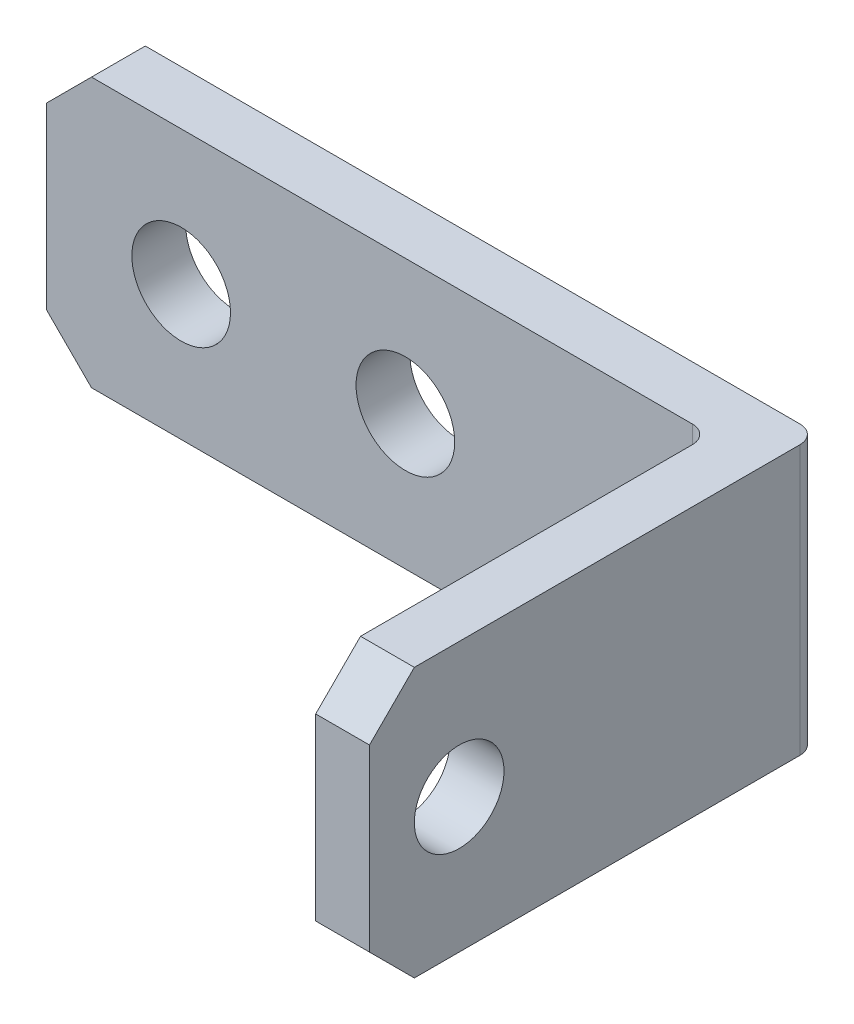
from build123d import *

# Parameters (mm, degrees)
SKETCH1_W           = 80
SKETCH1_H           = 30
SKETCH1_R           = 5.5
BOSS_EXTRUDE1_DEPTH = 6
SKETCH3_W           = 50
SKETCH3_H           = 30
SKETCH3_R           = 5
BOSS_EXTRUDE2_DEPTH = 6
FILLET1_R           = 2
CHAMFER1_SIZE       = 5


with BuildPart() as part:
    # Sketch1 → Boss-Extrude1 (new body)
    with BuildSketch(Plane.XY):
        Rectangle(SKETCH1_W, SKETCH1_H)
        Circle(SKETCH1_R, mode=Mode.SUBTRACT)
        with Locations((-25, 0)):
            Circle(SKETCH1_R, mode=Mode.SUBTRACT)
    extrude(amount=BOSS_EXTRUDE1_DEPTH)

    # Sketch3 → Boss-Extrude2 (add)
    with BuildSketch(Plane(origin=(40, 0, 0), x_dir=(0, 0, -1), z_dir=(1, 0, 0))):
        with Locations((-25, 0)):
            Rectangle(SKETCH3_W, SKETCH3_H)
        with Locations((-40, 0)):
            Circle(SKETCH3_R, mode=Mode.SUBTRACT)
    extrude(amount=-BOSS_EXTRUDE2_DEPTH)

    # Fillet1
    fillet1_edges = [part.edges().sort_by_distance(p)[0] for p in [
        (34, 0, 6),
        (40, 0, 0),
    ]]
    fillet(fillet1_edges, radius=FILLET1_R)

    # Chamfer1
    chamfer1_edges = [part.edges().sort_by_distance(p)[0] for p in [
        (37, 15, 50),
        (37, -15, 50),
        (-40, -15, 3),
        (-40, 15, 3),
    ]]
    chamfer(chamfer1_edges, length=CHAMFER1_SIZE)


solid = part.part
